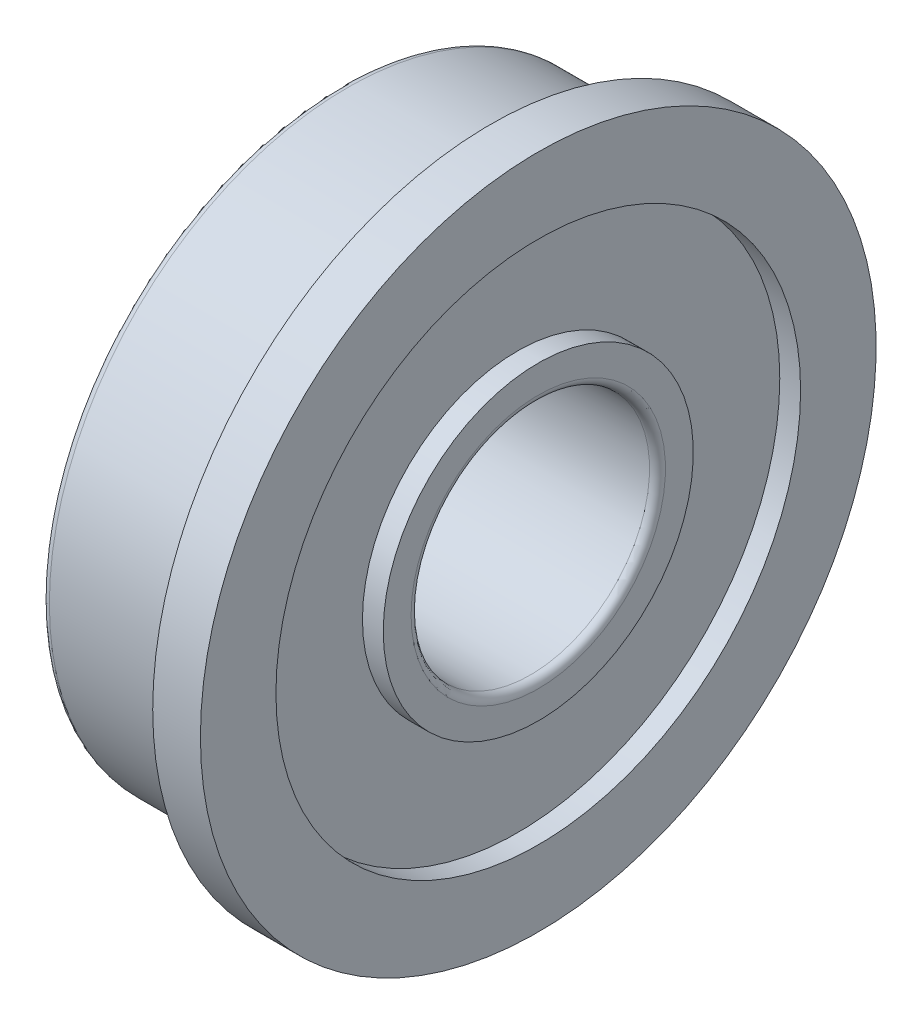
from build123d import *


with BuildPart() as part:
    # Sketch1 → Revolve1 (revolve)
    with BuildSketch(Plane.XY, mode=Mode.PRIVATE) as revolve1_sk:
        with BuildLine():
            Line((0, 7.3), (0, 6.6))
            Line((0, 6.6), (0.52375, 6.6))
            Line((0.52375, 6.6), (0.52375, 3.9))
            Line((0.52375, 3.9), (0, 3.9))
            Line((0, 3.9), (0, 3.2))
            ThreePointArc((0, 3.2), (0.058578644, 3.058578644), (0.2, 3))
            Line((0.2, 3), (4.8, 3))
            ThreePointArc((4.8, 3), (4.941421356, 3.058578644), (5, 3.2))
            Line((5, 3.2), (5, 3.9))
            Line((5, 3.9), (4.47625, 3.9))
            Line((4.47625, 3.9), (4.47625, 6.6))
            Line((4.47625, 6.6), (5, 6.6))
            Line((5, 6.6), (5, 8.5))
            Line((5, 8.5), (3.8, 8.5))
            Line((3.8, 8.5), (3.8, 7.7))
            ThreePointArc((3.8, 7.7), (3.941421356, 7.358578644), (3.6, 7.5))
            Line((3.6, 7.5), (0.2, 7.5))
            ThreePointArc((0.2, 7.5), (0.058578644, 7.441421356), (0, 7.3))
        make_face()
    revolve(revolve1_sk.sketch.rotate(Axis((15, 0, 0), (-1, 0, 0)), 270), axis=Axis((15, 0, 0), (-1, 0, 0)))


solid = part.part
